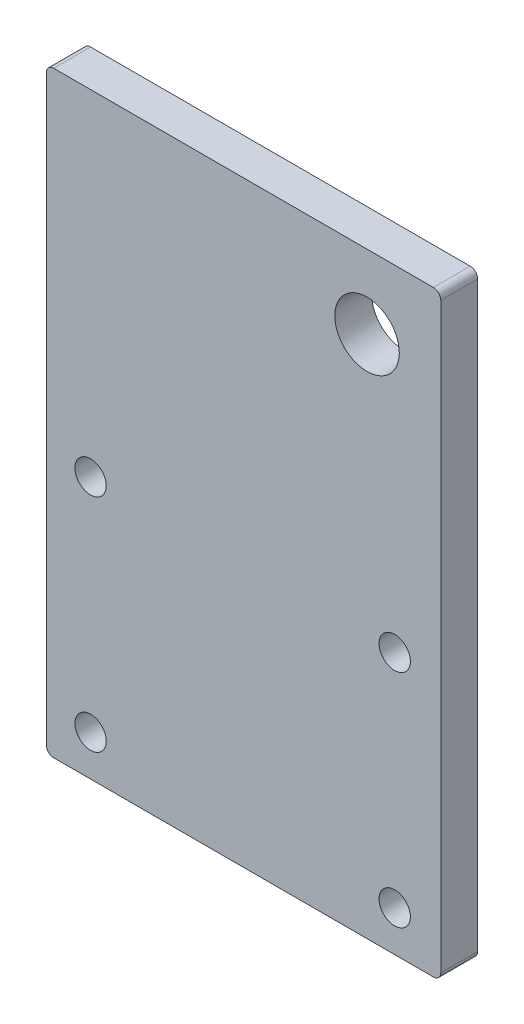
SolidWorks part; units mm, degrees
ref_plane "前视基准面" through (0, 0, 0) normal (0, 0, 1) x (1, 0, 0)
ref_plane "上视基准面" through (0, 0, 0) normal (0, 1, 0) x (1, 0, 0)
ref_plane "右视基准面" through (0, 0, 0) normal (1, 0, 0) x (0, 0, -1)
sketch "草图1" plane through (0, 0, 0) normal (0, 0, 1) x (1, 0, 0)
  line L1 (-53.5, -81) -> (53.5, -81)
  line L2 (-53.5, -81) -> (-53.5, 81)
  line L3 (-53.5, 81) -> (53.5, 81)
  line L4 (53.5, -81) -> (53.5, 81)
  line L5 (-53.5, -81) -> (53.5, 81) construction
  line L6 (-53.5, 81) -> (53.5, -81) construction
  point P0 (0, 0)
  dimension "D1" = 107
  dimension "D2" = 162
extrude "凸台-拉伸1" add sketch "草图1" along normal mid plane 10
hole_wizard "M20 螺纹孔1" positions "草图2" profile "草图3" tap size "M20" standard "GB" end condition through all
sketch "草图2" plane through (0, 0, 5) normal (0, 0, 1) x (1, 0, 0)
  line L2 (53.5, 81) -> (-53.5, 81) construction
  line L3 (53.5, -81) -> (53.5, 81) construction
  point P0 (33.5, 61)
  dimension "D1" = 20
  dimension "D2" = 20
sketch "草图3" plane through (33.5, 61, 5) normal (1, 0, 0) x (0, -1, 0)
  line L0 (0, 0) -> (0, 10)
  line L1 (0, 10) -> (8.75, 10)
  line L2 (8.75, 10) -> (8.75, 0)
  line L5 (8.75, 0) -> (0, 0)
  line L11 (0, -6.35) -> (0, 107.95) construction
  dimension "通孔螺纹孔钻头直径" = 17.5
  dimension "通孔螺纹孔钻头深度" = 10
cosmetic thread "孔螺蚊线1" parameters "D2"=20
fillet "圆角1" radius 2 4 edges at (-53.5, -81, 0) (53.5, -81, 0) (53.5, 81, 0) (-53.5, 81, 0)
hole_wizard "M10 螺纹孔1" positions "草图4" profile "草图5" tap size "M10" standard "GB" end condition through all
sketch "草图4" plane through (0, 0, 5) normal (0, 0, 1) x (1, 0, 0)
  line L0 (-51.5, -81) -> (51.5, -81) construction
  line L1 (-53.5, 79) -> (-53.5, -79) construction
  point P0 (-41.5, -70)
  dimension "D1" = 11
  dimension "D2" = 12
sketch "草图5" plane through (-41.5, -70, 5) normal (1, 0, 0) x (0, -1, 0)
  line L0 (0, 0) -> (0, 10)
  line L1 (0, 10) -> (4.25, 10)
  line L2 (4.25, 10) -> (4.25, 0)
  line L5 (4.25, 0) -> (0, 0)
  line L11 (0, -6.35) -> (0, 107.95) construction
  dimension "通孔螺纹孔钻头直径" = 8.5
  dimension "通孔螺纹孔钻头深度" = 10
cosmetic thread "孔螺蚊线2"
pattern_linear "阵列(线性)1" count 2 spacing 82.5 along (1, 0, 0) count 2 spacing 60 along (0, 1, 0) of "M10 螺纹孔1"
cosmetic thread "孔螺蚊线3"
cosmetic thread "孔螺蚊线4"
cosmetic thread "孔螺蚊线5"
